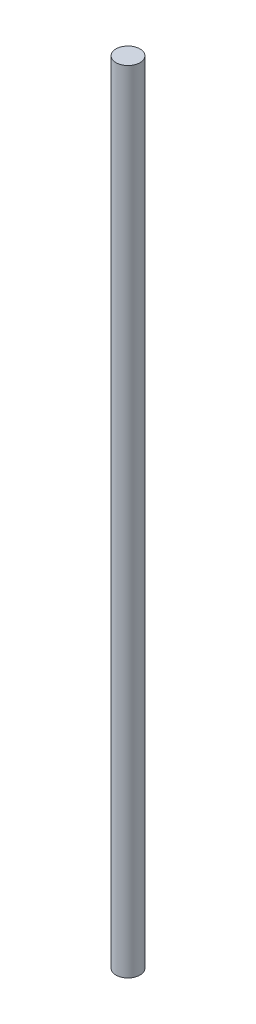
from build123d import *

# Parameters (mm, degrees)
SKETCH1_R           = 10
BOSS_EXTRUDE1_DEPTH = 660


with BuildPart() as part:
    # Sketch1 → Boss-Extrude1 (new body)
    with BuildSketch(Plane(origin=(0, 0, 0), x_dir=(1, 0, 0), z_dir=(0, 1, 0))):
        with Locations(Location((0, 0, 0), (0, 0, 270))):
            Circle(SKETCH1_R)
    extrude(amount=BOSS_EXTRUDE1_DEPTH)


solid = part.part
